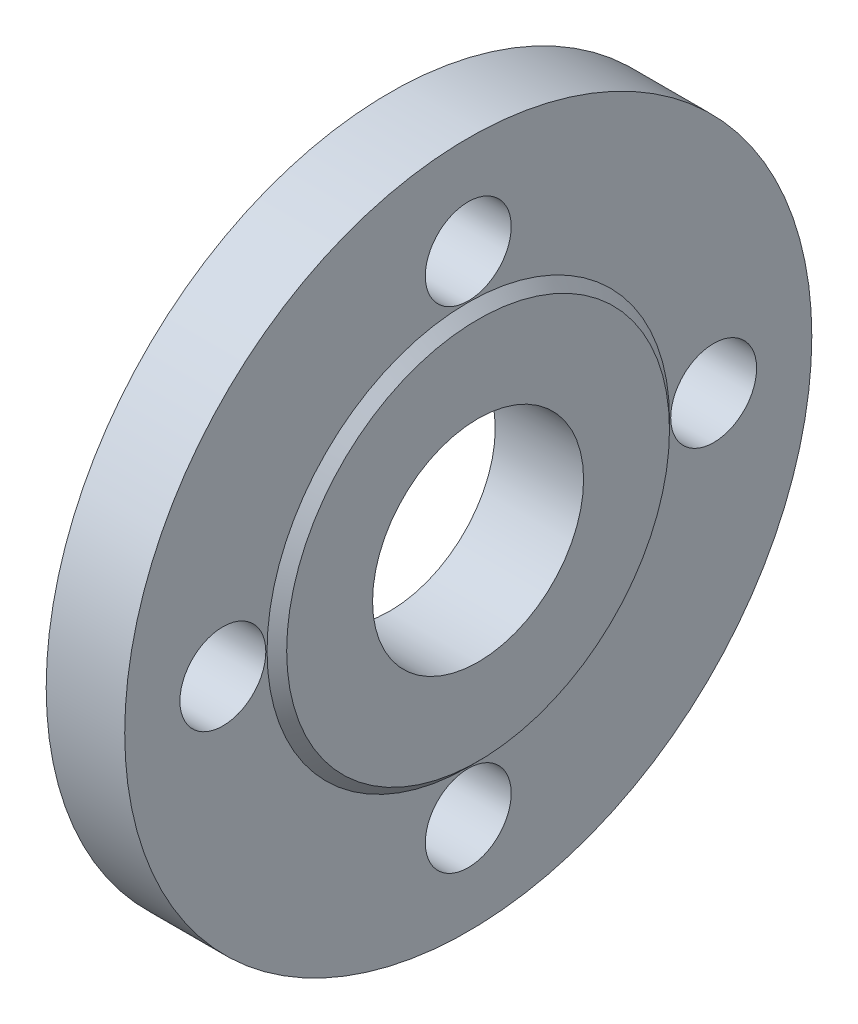
SolidWorks part; units mm, degrees
ref_plane "前视基准面" through (0, 0, 0) normal (0, 0, 1) x (1, 0, 0)
ref_plane "上视基准面" through (0, 0, 0) normal (0, 1, 0) x (1, 0, 0)
ref_plane "右视基准面" through (0, 0, 0) normal (1, 0, 0) x (0, 0, -1)
sketch "草图1" plane through (0, 0, 0) normal (0, 1, 0) x (1, 0, 0)
  line L0 (0, 21.5) -> (0, 70)
  line L1 (0, 70) -> (16, 70)
  line L2 (16, 70) -> (16, 41)
  line L3 (16, 41) -> (18, 39)
  line L4 (18, 39) -> (18, 21.5)
  line L5 (18, 21.5) -> (0, 21.5)
  line L6 (0, 0) -> (72.1913, 0) construction
  line L7 (0, 0) -> (0, 127.2752) construction
  dimension "D1" = 140
  dimension "D2" = 43
  dimension "D3" = 78
  dimension "D4" = 2
  dimension "D5" = 18
  dimension "D6" = 2
revolve "旋转1" add sketch "草图1" angle 360 about L6
sketch "草图2" plane through (16, 0, 0) normal (1, 0, 0) x (0, 0, -1)
  line L0 (0, 0) -> (0, 50) construction
  circle A0 centre (0, 50) radius 8.75
  circle A1 centre (0, 0) radius 50 construction
  circle A2 centre (50, 0) radius 8.75
  circle A3 centre (0, -50) radius 8.75
  circle A4 centre (-50, 0) radius 8.75
  point P5 (-52.5827, -2.6395)
  point P6 (0, 0)
  point P14 (0, 0)
  dimension "D1" = 100
  dimension "D2" = 17.5
  dimension "D3" = 4
extrude "切除-拉伸1" cut sketch "草图2" against normal through all both and the other way through all
